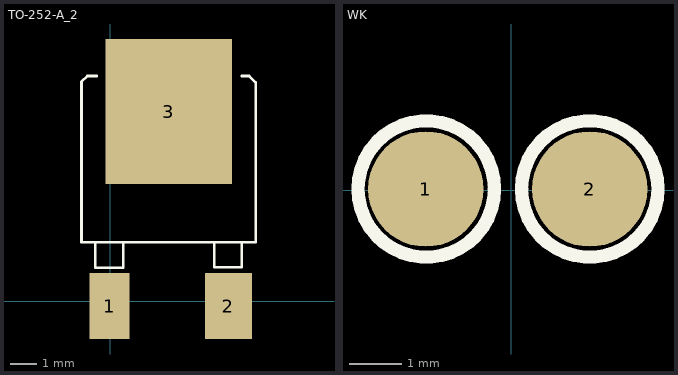
[diagram p0: the footprints below, top view; thin cyan lines are the x and y axes]
# Altium footprint library MISC86331.PcbLib: 18 footprints (part 2 of 2)
Each footprint in its own frame and in the unit in brackets; x right, y up, seen from the top. Pads: shape width x height; smd on the part's side, far side on the other; paste and mask are expansions set on the pad; w line width, h text height; cw(c..) or ccw(c..) is an arc to the next point about the centre after c.

## TO-252-A_2 [mm]
pads (3):
  rect 1.5x2.5 smd: 1(-0.026,-0.189)
  rect 1.8x2.5 smd: 2(4.484,-0.189)
  rect 4.8x5.5 smd: 3(2.214,7.181)
Top Overlay:
  lines w0.1: -0.561,2.231 -0.561,1.256 0.489,1.256 0.489,2.181 ; -0.511,8.531 -0.869,8.531 -1.086,8.314 -1.086,2.231 5.514,2.231 5.514,8.286 5.269,8.531 4.989,8.531 ; 3.939,2.231 3.939,1.281 4.989,1.281 4.989,2.231
3D body: height 0.5, standoff 0, extent -0.95,8.1 5.25,9.65
3D body: height 0.5, standoff 0, extent -0.6,-0.25 0.45,2.25
3D body: height 0.5, standoff 0, extent 3.9,-0.35 4.95,2.15
3D body: height 0.5, standoff 0, extent 1.6,1.3 2.65,2.55
3D body: height 0.5, standoff 0, extent -0.95,2.3 5.35,8.25
3D body: height 2.5, standoff 0, extent -0.95,8.05 -0.95,8.15

## WK [mm]
height 2.45
pads (2):
  round 2.2 smd: 1(-1.625,0.025) 2(1.5,0.025)
Top Overlay:
  circle w0.254: c1.5,0.025 r1.3
  circle w0.254: c-1.618,0.025 r1.3